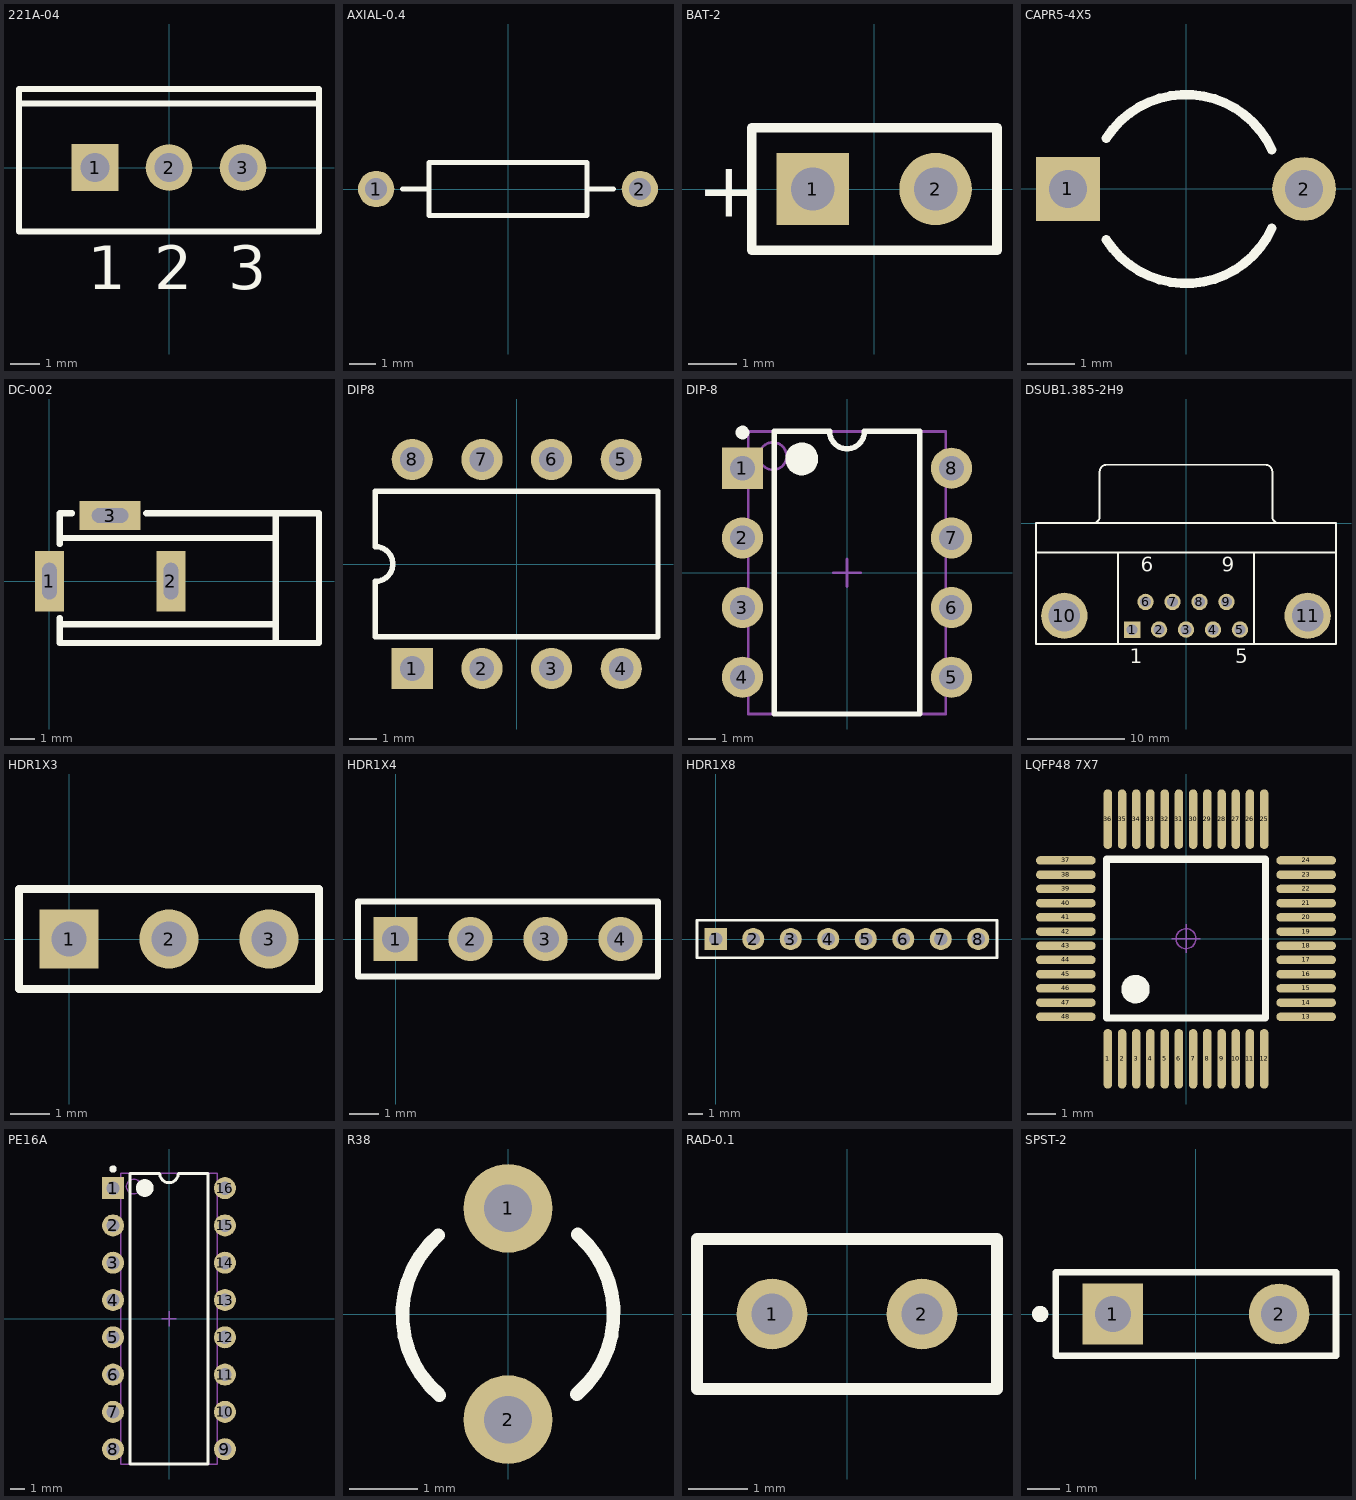
[diagram p0: the footprints below, top view; thin cyan lines are the x and y axes]
# Altium footprint library MISC84364-8.PcbLib: 16 footprints
Each footprint in its own frame and in the unit in brackets; x right, y up, seen from the top. Pads: shape width x height; smd on the part's side, far side on the other; paste and mask are expansions set on the pad; w line width, h text height; cw(c..) or ccw(c..) is an arc to the next point about the centre after c.

## 221A-04 [mm]
pads (3):
  rect 1.6x1.6 hole 1: 1(-2.54,0)
  round 1.6 hole 1: 2(0,0) 3(2.54,0)
Top Overlay:
  lines w0.2: -5.15,2.2 5.15,2.2 ; -5.15,-2.2 -5.15,2.7 5.15,2.7 5.15,-2.2 -5.15,-2.2
  text "3" at 2.04,-4.175 h1.5
  text "2" at -0.5,-4.175 h1.5
  text "1" at -2.79,-4.175 h1.5

## AXIAL-0.4 [mm]
pads (2):
  round 1.4 hole 0.85: 1(-5.08,0) 2(5.08,0)
Top Overlay:
  lines w0.2: -4.064,0 -3.048,0 ; 3.048,0 4.064,0 ; -3.048,-1.016 -3.048,1.016 3.048,1.016 3.048,-1.016 -3.048,-1.016

## BAT-2 [mm]
pads (2):
  rect 1.5x1.5 hole 0.9: 1(-1.27,0)
  round 1.5 hole 0.9: 2(1.27,0)
Top Overlay:
  lines w0.2: -2.54,-1.27 -2.54,1.27 2.54,1.27 2.54,-1.27 -2.54,-1.27
  text "+" at -3.67,-0.577 h1.15

## CAPR5-4X5 [mm]
pads (2):
  rect 1.35x1.35 hole 0.8: 1(-2.5,0)
  round 1.35 hole 0.8: 2(2.5,0)
Top Overlay:
  lines w0.2: -1.687,-1.075 ccw(c0,0) 1.819,-0.832 ; -1.687,1.075 cw(c0,0) 1.819,0.832

## DC-002 [mm]
pads (3):
  rect 1.2x2.5 hole 0.6 slot 1.5 at 90 deg: 1(0,0) 2(5,0)
  rect 2.5x1.2 hole 0.6 slot 1.5 at 0 deg: 3(2.5,2.7)
Top Overlay:
  lines w0.254: 0.428,-1.778 9.318,-1.778 ; 0.428,-1.524 0.428,-2.54 11.096,-2.54 11.096,2.794 3.984,2.794 ; 0.428,1.524 0.428,2.794 0.936,2.794 ; 0.428,1.778 9.318,1.778 ; 9.318,-2.54 9.318,-1.778 ; 9.318,2.794 9.318,1.778 ; 9.318,-1.778 9.318,1.778
3D body "DC-002.STEP": height 7.3, standoff -3.4, extent -0.254,-2.548 11.046,2.802

## DIP8 [mm]
pads (8):
  rect 1.5x1.5 hole 0.9: 1(-3.81,-3.81)
  round 1.5 hole 0.9: 2(-1.27,-3.81) 3(1.27,-3.81) 4(3.81,-3.81) 5(3.81,3.81) 6(1.27,3.81) 7(-1.27,3.81) 8(-3.81,3.81)
Top Overlay:
  lines w0.2: -5.15,-2.65 5.15,-2.65 5.15,2.65 -5.15,2.65 -5.15,0.635 cw(c-5.15,0) -5.15,-0.635 -5.15,-2.65

## DIP-8 [mm]
pads (8):
  rect 1.5x1.5 hole 0.9: 1(-3.81,3.81)
  round 1.5 hole 0.9: 2(-3.81,1.27) 3(-3.81,-1.27) 4(-3.81,-3.81) 5(3.81,-3.81) 6(3.81,-1.27) 7(3.81,1.27) 8(3.81,3.81)
Top Overlay:
  circle w0.25: c-3.81,5.11 r0.125
  circle w0.6: c-1.65,4.15 r0.3
  lines w0.2: -2.65,-5.15 -2.65,5.15 -0.635,5.15 ccw(c0,5.15) 0.635,5.15 2.65,5.15 2.65,-5.15 -2.65,-5.15
Mechanical 13:
  circle w0.1: c-2.7,4.25 r0.5
  lines w0.1: -3.6,-5.15 -3.6,5.15 3.6,5.15 3.6,-5.15 -3.6,-5.15
Mechanical 15:
  lines w0.1: -0.5,0 0.5,0 ; 0,-0.5 0,0.5
3D body: height 5.08, standoff 0, extent -3.6,-5.15 3.6,5.15

## DSUB1.385-2H9 [mm]
pads (11):
  rect 1.69x1.69 hole 1.09: 1(-5.54,-10.92)
  round 1.69 hole 1.09: 2(-2.77,-10.92) 3(0,-10.92) 4(2.77,-10.92) 5(5.54,-10.92) 6(-4.155,-8.08) 7(-1.385,-8.08) 8(1.385,-8.08) 9(4.155,-8.08)
  round 4.76 hole 3.26: 10(-12.495,-9.5) 11(12.495,-9.5)
Top Overlay:
  lines w0.2: -15.4,-3 15.4,-3 ; -9.56,0.005 ccw(c-9.56,0.7) -8.865,0.7 -8.865,5.3 ; -8.86,5.305 cw(c-8.165,5.305) -8.165,6 8.165,6 cw(c8.165,5.305) 8.86,5.305 ; -7,-12.4 -7,-3 ; 7,-12.4 7,-3 ; 8.865,5.3 8.865,0.7 ccw(c9.56,0.7) 9.56,0.005 ; -15.4,-12.4 15.4,-12.4 15.4,0 -15.4,0 -15.4,-12.4
  text "6" at -4.655,-4.975 h1.5
  text "9" at 3.655,-4.975 h1.5
  text "5" at 5.04,-14.375 h1.5
  text "1" at -5.79,-14.375 h1.5

## HDR1X3 [mm]
pads (3):
  rect 1.5x1.5 hole 0.9: 1(0,0)
  round 1.5 hole 0.9: 2(2.54,0) 3(5.08,0)
Top Overlay:
  lines w0.2: -1.27,-1.27 6.35,-1.27 6.35,1.27 -1.27,1.27 -1.27,-1.27

## HDR1X4 [mm]
pads (4):
  rect 1.5x1.5 hole 0.9: 1(0,0)
  round 1.5 hole 0.9: 2(2.54,0) 3(5.08,0) 4(7.62,0)
Top Overlay:
  lines w0.2: -1.27,-1.27 -1.27,1.27 8.89,1.27 8.89,-1.27 -1.27,-1.27

## HDR1X8 [mm]
pads (8):
  rect 1.5x1.5 hole 0.9: 1(0,0)
  round 1.5 hole 0.9: 2(2.54,0) 3(5.08,0) 4(7.62,0) 5(10.16,0) 6(12.7,0) 7(15.24,0) 8(17.78,0)
Top Overlay:
  lines w0.2: -1.27,-1.27 19.05,-1.27 19.05,1.27 -1.27,1.27 -1.27,-1.27

## LQFP48 7X7 [mm]
pads (48):
  oval 0.3x2.1 smd: 1(-2.75,-4.227) 2(-2.25,-4.227) 3(-1.75,-4.227) 4(-1.25,-4.227) 5(-0.75,-4.227) 6(-0.25,-4.227) 7(0.25,-4.227) 8(0.75,-4.227) 9(1.25,-4.227) 10(1.75,-4.227) 11(2.25,-4.227) 12(2.75,-4.227) 25(2.75,4.202) 26(2.25,4.202) 27(1.75,4.202) 28(1.25,4.202) 29(0.75,4.202) 30(0.25,4.202) 31(-0.25,4.202) 32(-0.75,4.202) 33(-1.25,4.202) 34(-1.75,4.202) 35(-2.25,4.202) 36(-2.75,4.202)
  oval 2.1x0.3 smd: 13(4.227,-2.75) 14(4.227,-2.25) 15(4.227,-1.75) 16(4.227,-1.25) 17(4.227,-0.75) 18(4.227,-0.25) 19(4.227,0.25) 20(4.227,0.75) 21(4.227,1.25) 22(4.227,1.75) 23(4.227,2.25) 24(4.227,2.75) 37(-4.227,2.75) 38(-4.227,2.25) 39(-4.227,1.75) 40(-4.227,1.25) 41(-4.227,0.75) 42(-4.227,0.25) 43(-4.227,-0.25) 44(-4.227,-0.75) 45(-4.227,-1.25) 46(-4.227,-1.75) 47(-4.227,-2.25) 48(-4.227,-2.75)
Top Overlay:
  circle w0.5: c-1.778,-1.778 r0.25
  lines w0.254: -2.794,-2.794 2.794,-2.794 2.794,2.794 -2.794,2.794 -2.794,-2.794
Mechanical 15:
  circle w0.05: c0,0 r0.35
  lines w0.05: -0.5,0 0.5,0 ; 0,-0.5 0,0.5
3D body "LQFP48 7X7.STEP": height 1.45, standoff 0, extent -4.51,-4.503 4.496,4.503

## PE16A [mm]
pads (16):
  rect 1.5x1.5 hole 0.9: 1(-3.81,8.89)
  round 1.5 hole 0.9: 2(-3.81,6.35) 3(-3.81,3.81) 4(-3.81,1.27) 5(-3.81,-1.27) 6(-3.81,-3.81) 7(-3.81,-6.35) 8(-3.81,-8.89) 9(3.81,-8.89) 10(3.81,-6.35) 11(3.81,-3.81) 12(3.81,-1.27) 13(3.81,1.27) 14(3.81,3.81) 15(3.81,6.35) 16(3.81,8.89)
Top Overlay:
  circle w0.6: c-1.65,8.9 r0.3
  circle w0.25: c-3.81,10.19 r0.125
  lines w0.2: -2.65,-9.9 2.65,-9.9 2.65,9.9 0.635,9.9 cw(c0,9.9) -0.635,9.9 -2.65,9.9 -2.65,-9.9
Mechanical 13:
  circle w0.1: c-2.4,9 r0.5
  lines w0.1: -3.3,-9.9 3.3,-9.9 3.3,9.9 -3.3,9.9 -3.3,-9.9
Mechanical 15:
  lines w0.1: -0.5,0 0.5,0 ; 0,-0.5 0,0.5
3D body: height 5.08, standoff 0, extent -3.3,-9.9 3.3,9.9

## R38 [mm]
pads (2):
  round 1.3 hole 0.7: 1(0,1.55) 2(0,-1.55)
Top Overlay:
  lines w0.2: -1.022,1.155 ccw(c0,-0.01) -1.006,-1.189 ; 1.006,-1.179 ccw(c0,0) 1.022,1.165

## RAD-0.1 [mm]
pads (2):
  round 1.2 hole 0.7: 1(-1.27,0) 2(1.27,0)
Top Overlay:
  lines w0.2: -2.54,-1.27 -2.54,1.27 2.54,1.27 2.54,-1.27 -2.54,-1.27

## SPST-2 [mm]
pads (2):
  rect 1.85x1.85 hole 1.1: 1(-2.54,0)
  round 1.85 hole 1.1: 2(2.54,0)
Top Overlay:
  circle w0.25: c-4.761,-0.001 r0.125
  lines w0.2: -4.28,-1.27 4.28,-1.27 4.28,1.27 -4.28,1.27 -4.28,-1.27